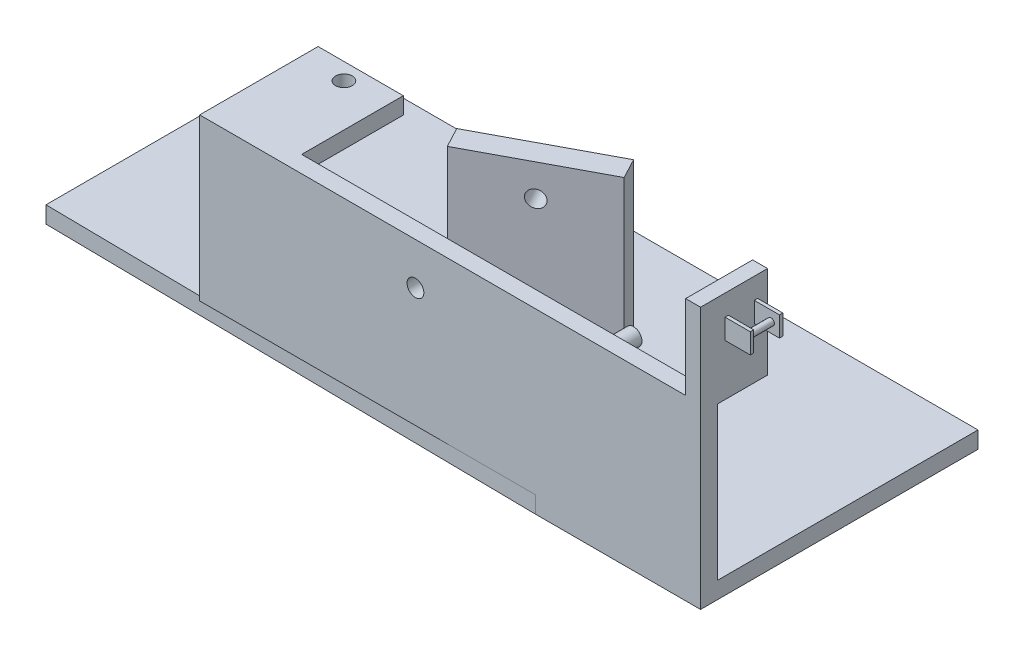
SolidWorks part; units mm, degrees
material "PBT general purpose"
ref_plane "Front Plane" through (0, 0, 0) normal (0, 0, 1) x (1, 0, 0)
ref_plane "Top Plane" through (0, 0, 0) normal (0, 1, 0) x (1, 0, 0)
ref_plane "Right Plane" through (0, 0, 0) normal (1, 0, 0) x (0, 0, -1)
sketch "Sketch1" plane through (0, 0, 0) normal (0, 1, 0) x (1, 0, 0)
  line L0 (-110.4399, 19.8241) -> (89.5601, 19.8241)
  line L1 (-120.4399, -55.1759) -> (99.5601, -55.1759)
  line L2 (-120.4399, -55.1759) -> (-120.4399, 29.8241)
  line L3 (-120.4399, 29.8241) -> (99.5601, 29.8241)
  line L4 (99.5601, -55.1759) -> (99.5601, 29.8241)
  line L5 (89.5601, -45.1759) -> (89.5601, 19.8241)
  line L6 (-110.4399, -45.1759) -> (89.5601, -45.1759)
  line L7 (-110.4399, -45.1759) -> (-110.4399, 19.8241)
  dimension "D2" = 65
  dimension "D3" = 200
  dimension "D1" = 10
extrude "Boss-Extrude1" add sketch "Sketch1" along normal blind 50
sketch "Sketch2" plane through (0, 0, 55.1759) normal (0, 0, 1) x (1, 0, 0)
  line L0 (-120.4399, 50) -> (-120.4399, 0) construction
  circle A0 centre (-70.4399, 25) radius 5
  point P2 (-120.4399, 25)
  dimension "D1" = 10
  dimension "D2" = 50
extrude "Cut-Extrude1" cut sketch "Sketch2" against normal up to surface (85 mm away) up to face at (-10.4399, 25, -29.8241)
sketch "Sketch3" plane through (0, 0, 55.1759) normal (0, 0, 1) x (1, 0, 0)
  circle A0 centre (-16.4399, 25) radius 5
  circle A1 centre (-70.4399, 25) radius 5 construction
  dimension "D1" = 10
  dimension "D2" = 54
extrude "Boss-Extrude2" add sketch "Sketch3" against normal up to surface (75 mm away) up to face at (-65.4399, 25, -19.8241)
sketch "Sketch4" plane through (0, 0, 55.1759) normal (0, 0, 1) x (1, 0, 0)
  line L0 (-120.4399, 50) -> (-120.4399, 87.8143)
  line L1 (-120.4399, 87.8143) -> (-48.8108, 87.8143)
  line L2 (-48.8108, 87.8143) -> (-48.8108, 77.8143)
  line L3 (-48.8108, 77.8143) -> (-110.4399, 77.8143)
  line L4 (-110.4399, 77.8143) -> (-110.4399, 50)
  line L5 (-120.4399, 50) -> (99.5601, 50) construction
  line L6 (-110.4399, 50) -> (-120.4399, 50)
  dimension "D1" = 10
  dimension "D2" = 10
extrude "Boss-Extrude3" add sketch "Sketch4" against normal up to surface (85 mm away) up to face at (-65.4399, 25, -29.8241)
sketch "Sketch7" plane through (0, 0, 55.1759) normal (0, 0, 1) x (1, 0, 0)
  line L0 (-120.4399, 0) -> (99.5601, 0) construction
  line L1 (-110.4399, 0) -> (99.5601, 0)
  line L2 (-110.4399, 0) -> (-110.4399, 50)
  line L3 (-110.4399, 50) -> (99.5601, 50)
  line L4 (99.5601, 0) -> (99.5601, 50)
extrude "Cut-Extrude3" cut sketch "Sketch7" against normal blind 35
sketch "Sketch8" plane through (89.5601, 0, 0) normal (-1, 0, 0) x (0, 0, 1)
  line L0 (20.1759, 50) -> (-19.8241, 50) construction
  line L1 (20.1759, 0) -> (10.1759, 0)
  line L2 (20.1759, 0) -> (20.1759, 50)
  line L3 (20.1759, 50) -> (10.1759, 50)
  line L4 (10.1759, 0) -> (10.1759, 50)
  dimension "D1" = 10
extrude "Boss-Extrude4" add sketch "Sketch8" along normal up to surface (200 mm away) up to face at (-110.4399, 42.6048, 1.0092)
sketch "Sketch9" plane through (0, 0, 0) normal (0, -1, 0) x (1, 0, 0)
  line L0 (-110.4399, 20.1759) -> (99.5601, 20.1759) construction
  line L1 (99.5601, -29.8241) -> (24.7244, -29.8241)
  line L2 (99.5601, -29.8241) -> (99.5601, 20.1759)
  line L3 (99.5601, 20.1759) -> (24.7244, 20.1759)
  line L4 (24.7244, -29.8241) -> (24.7244, 20.1759)
extrude "Boss-Extrude5" add sketch "Sketch9" against normal blind 5
sketch "Sketch10" plane through (0, 50, 0) normal (0, 1, 0) x (1, 0, 0)
  line L0 (99.5601, 29.8241) -> (-110.4399, 29.8241) construction
  line L1 (99.5601, -20.1759) -> (46.5233, -20.1759)
  line L2 (99.5601, -20.1759) -> (99.5601, 29.8241)
  line L3 (99.5601, 29.8241) -> (46.5233, 29.8241)
  line L4 (46.5233, -20.1759) -> (46.5233, -2.1759)
  line L5 (46.5233, -2.1759) -> (54.5601, -2.1759)
  line L6 (54.5601, -2.1759) -> (54.5601, 9.8241)
  line L7 (54.5601, 9.8241) -> (46.5233, 9.8241)
  line L8 (46.5233, 9.8241) -> (46.5233, 29.8241)
  dimension "D1" = 18
  dimension "D2" = 12
  dimension "D3" = 45
extrude "Boss-Extrude6" add sketch "Sketch10" against normal blind 5
sketch "Sketch11" plane through (0, 50, 0) normal (0, 1, 0) x (1, 0, 0)
  line L0 (99.5601, 29.8241) -> (-110.4399, 29.8241) construction
  line L1 (99.5601, -20.1759) -> (63.4572, -20.1759)
  line L2 (99.5601, -20.1759) -> (99.5601, 29.8241)
  line L3 (99.5601, 29.8241) -> (63.4572, 29.8241)
  line L4 (63.4572, -20.1759) -> (63.4572, 29.8241)
extrude "Cut-Extrude4" cut sketch "Sketch11" against normal through all
sketch "Sketch12" plane through (0, 50, 0) normal (0, 1, 0) x (1, 0, 0)
  line L0 (63.4572, 29.8241) -> (63.4572, -20.1759) construction
  line L1 (46.5233, -10.1759) -> (63.4572, -10.1759)
  line L2 (46.5233, -10.1759) -> (46.5233, -2.1759)
  line L3 (46.5233, 19.755) -> (63.4572, 19.755)
  line L4 (63.4572, -10.1759) -> (63.4572, 19.755)
  line L5 (46.5233, 9.8241) -> (46.5233, 19.755)
  line L6 (54.5601, -2.1759) -> (46.5233, -2.1759)
  line L7 (54.5601, -2.1759) -> (54.5601, 9.8241)
  line L8 (54.5601, 9.8241) -> (46.5233, 9.8241)
extrude "Boss-Extrude7" add sketch "Sketch12" along normal blind 50
sketch "Sketch13" plane through (0, 0, 0) normal (0, -1, 0) x (1, 0, 0)
  line L0 (-120.4399, 55.1759) -> (-120.4399, 105.1759)
  line L2 (-110.4399, 108.1048) -> (-62.671, 155.8738)
  line L3 (-62.671, 155.8738) -> (-66.2065, 159.4093)
  line L4 (-110.4399, 108.1048) -> (-110.4399, 55.1759)
  line L5 (-48.8108, 55.1759) -> (-120.4399, 55.1759) construction
  line L6 (-110.4399, 55.1759) -> (-120.4399, 55.1759)
  line L7 (-66.2065, 159.4093) -> (-120.4399, 105.1759)
  dimension "D1" = 5
  dimension "D2" = 10
  dimension "D3" = 135
extrude "Boss-Extrude8" add sketch "Sketch13" against normal blind 50 separate body
sketch "Sketch14" plane through (0, 0, 10.1759) normal (0, 0, -1) x (-1, 0, 0)
  circle A0 centre (70.4399, 25) radius 4.9995
extrude "Cut-Extrude5" cut sketch "Sketch14" against normal blind 50
sketch "Sketch17" plane through (0, 0, 0) normal (0, -1, 0) x (1, 0, 0)
  line L0 (24.7244, -19.8241) -> (-110.4399, -19.8241) construction
  line L1 (63.4572, -29.8241) -> (-110.4399, -29.8241)
  line L2 (63.4572, -29.8241) -> (63.4572, -19.8241)
  line L3 (63.4572, -19.8241) -> (-110.4399, -19.8241)
  line L4 (-110.4399, -29.8241) -> (-110.4399, -19.8241)
extrude "Cut-Extrude7" cut sketch "Sketch17" against normal up to next (50 mm away)
sketch "Sketch18" plane through (-109.2724, 0, 109.2724) normal (0.7071, 0, -0.7071) x (-0.7071, 0, -0.7071)
  line L0 (1.6512, 0) -> (-65.9043, 0) construction
  circle A0 centre (-32.1266, 25) radius 5
  dimension "D1" = 10
  dimension "D2" = 25
extrude "Cut-Extrude8" cut sketch "Sketch18" against normal blind 10
sketch "Sketch20" plane through (0, 87.8143, 0) normal (0, 1, 0) x (1, 0, 0)
  circle A0 centre (-70.1737, -35.2467) radius 5
extrude "Cut-Extrude9" cut sketch "Sketch20" against normal blind 15
sketch "Sketch23" plane through (0, 0, 0) normal (0, -1, 0) x (1, 0, 0)
  line L1 (24.7244, 10.1759) -> (63.4572, 10.1759)
  line L2 (24.7244, 10.1759) -> (24.7244, -19.8241)
  line L3 (24.7244, -19.8241) -> (63.4572, -19.8241)
  line L4 (63.4572, 10.1759) -> (63.4572, -19.8241)
extrude "Cut-Extrude12" cut sketch "Sketch23" against normal blind 15
sketch "Sketch24" plane through (-110.4399, 0, 0) normal (1, 0, 0) x (0, 0, -1)
  line L1 (-178.5753, 76.7479) -> (-55.1759, 76.7479)
  line L2 (-178.5753, 76.7479) -> (-178.5753, 0)
  line L3 (-178.5753, 0) -> (-55.1759, 0)
  line L4 (-55.1759, 76.7479) -> (-55.1759, 0)
extrude "Cut-Extrude14" cut sketch "Sketch24" against normal mid plane 100
sketch "Sketch26" plane through (0, 0, 0) normal (0, -1, 0) x (1, 0, 0)
  line L0 (-120.4399, -29.8241) -> (-120.4399, -82.8241)
  line L1 (-110.4399, -29.8241) -> (-110.4399, -82.8241)
  line L2 (-110.4399, -82.8241) -> (-60.5112, -132.7528)
  line L3 (-120.4399, -82.8241) -> (-64.6115, -138.6525)
  line L4 (-64.6115, -138.6525) -> (-60.5112, -132.7528)
  line L5 (-120.4399, -29.8241) -> (-110.4399, -29.8241)
extrude "Boss-Extrude9" add sketch "Sketch26" against normal blind 60
sketch "Sketch27" plane through (-96.632, 0, -96.632) normal (0.7071, 0, 0.7071) x (0.7071, 0, -0.7071)
  circle A0 centre (14.4727, 25) radius 5
extrude "Cut-Extrude15" cut sketch "Sketch27" against normal blind 60
sketch "Sketch28" plane through (63.4572, 0, 0) normal (1, 0, 0) x (0, 0, -1)
  line L4 (-3.5599, 87.5411) -> (-5.5599, 87.5411)
  line L5 (-5.5599, 87.5411) -> (-5.5599, 75.5411)
  line L6 (-3.5599, 87.5411) -> (-3.5599, 75.5411)
  line L7 (-3.5599, 75.5411) -> (-5.5599, 75.5411)
  line L8 (11.8241, 87.5411) -> (13.8241, 87.5411)
  line L9 (13.8241, 87.5411) -> (13.8241, 75.5411)
  line L10 (13.8241, 75.5411) -> (11.8241, 75.5411)
  line L11 (11.8241, 75.5411) -> (11.8241, 87.5411)
extrude "Boss-Extrude10" add sketch "Sketch28" along normal blind 15
sketch "Sketch29" plane through (0, 0, 5.5599) normal (0, 0, 1) x (1, 0, 0)
  circle A0 centre (73.4572, 81.5411) radius 2
extrude "Boss-Extrude11" add sketch "Sketch29" against normal blind 18
sketch "Sketch30" plane through (-48.8108, 0, 0) normal (1, 0, 0) x (0, 0, -1)
  line L0 (10.1347, 87.8143) -> (18.6732, 87.8143)
  line L1 (29.8241, 87.8143) -> (-55.1759, 87.8143) construction
  line L2 (18.6732, 87.8143) -> (14.404, 97.0575)
  line L3 (14.404, 97.0575) -> (10.1347, 87.8143)
sketch "Sketch31" plane through (0, 87.8143, 0) normal (0, 1, 0) x (1, 0, 0)
  line L0 (-48.8108, 10.1347) -> (-48.8108, 18.6732) construction
  line L1 (-120.4399, 29.8241) -> (-120.4399, -55.1759) construction
  spline S0 degree 3 poles (-48.8108, 14.404) (-68.2087, 19.7403) (-84.0911, -3.4277) (-107.8721, -25.1931) (-120.4399, -12.6759) knots 0 0 0 0 0.557371 1 1 1 1
sweep "Sweep1" add profiles "Sketch30" path "Sketch31"
sketch "Sketch32" plane through (-110.4399, 0, 0) normal (1, 0, 0) x (0, 0, -1)
  line L1 (29.8241, 60) -> (152.1894, 60)
  line L2 (29.8241, 60) -> (29.8241, -15.4022)
  line L3 (29.8241, -15.4022) -> (152.1894, -15.4022)
  line L4 (152.1894, 60) -> (152.1894, -15.4022)
extrude "Cut-Extrude16" cut sketch "Sketch32" against normal mid plane 100
sketch "Sketch33" plane through (0, 0, -9.8241) normal (0, 0, 1) x (1, 0, 0)
  line L1 (54.5601, 100) -> (46.5233, 100)
  line L2 (54.5601, 100) -> (54.5601, 45)
  line L3 (54.5601, 45) -> (46.5233, 45)
  line L4 (46.5233, 100) -> (46.5233, 45)
extrude "Cut-Extrude17" cut sketch "Sketch33" against normal mid plane 40
sketch "Sketch34" plane through (0, 0, 10.1759) normal (0, 0, 1) x (1, 0, 0)
  line L1 (54.5601, 100) -> (63.4572, 100)
  line L2 (54.5601, 100) -> (54.5601, 50)
  line L3 (54.5601, 50) -> (63.4572, 50)
  line L4 (63.4572, 100) -> (63.4572, 50)
extrude "Boss-Extrude12" add sketch "Sketch34" along normal blind 10
sketch "Sketch35" plane through (0, 0, -19.8241) normal (0, 0, -1) x (-1, 0, 0)
  line L0 (16.4399, 25) -> (16.4399, -46)
ref_plane "Plane1" through (0, -46, 0) normal (0, 1, 0) x (1, 0, 0)
sketch "Sketch36" plane through (0, -46, 0) normal (0, 1, 0) x (1, 0, 0)
  line L0 (-110.4399, -20.1759) -> (63.4572, -20.1759) construction
  line L1 (-35.0234, -20.1759) -> (63.4572, -20.1759)
  line L2 (-35.0234, -20.1759) -> (-35.0234, 30.7287)
  line L3 (-35.0234, 30.7287) -> (63.4572, 30.7287)
  line L4 (63.4572, -20.1759) -> (63.4572, 30.7287)
extrude "Boss-Extrude13" add sketch "Sketch36" against normal blind 10 separate body
sketch "Sketch37" plane through (0, -46, 0) normal (0, 1, 0) x (1, 0, 0)
  line L0 (63.4572, -20.1759) -> (63.4572, 30.7287) construction
  line L1 (-35.0234, -20.1759) -> (63.4572, -20.1759)
  line L2 (-35.0234, -20.1759) -> (-35.0234, -10.1759)
  line L3 (-35.0234, -10.1759) -> (63.4572, -10.1759)
  line L4 (63.4572, -20.1759) -> (63.4572, -10.1759)
  line L5 (-110.4399, -10.1759) -> (63.4572, -10.1759) construction
extrude "Boss-Extrude14" add sketch "Sketch37" along normal blind 46
ref_plane "Plane2" through (-35.0234, 0, 0) normal (1, 0, 0) x (0, 0, -1)
sketch "Sketch39" plane through (-35.0234, 0, 0) normal (1, 0, 0) x (0, 0, -1)
  line L1 (35.5386, 90.5816) -> (-64.8845, 90.5816)
  line L2 (35.5386, 90.5816) -> (35.5386, -58.8284)
  line L3 (35.5386, -58.8284) -> (-64.8845, -58.8284)
  line L4 (-64.8845, 90.5816) -> (-64.8845, -58.8284)
extrude "Cut-Extrude21" cut sketch "Sketch39" against normal blind 100
sketch "Sketch40" plane through (-35.0234, 0, 0) normal (1, 0, 0) x (0, 0, -1)
  line L1 (-73.704, 85.0863) -> (47.7926, 85.0863)
  line L2 (-73.704, 85.0863) -> (-73.704, 128.8491)
  line L3 (-73.704, 128.8491) -> (47.7926, 128.8491)
  line L4 (47.7926, 85.0863) -> (47.7926, 128.8491)
extrude "Cut-Extrude22" cut sketch "Sketch40" against normal blind 100
ref_plane "Plane3" through (0, -56, 0) normal (0, 1, 0) x (1, 0, 0)
sketch "Sketch41" plane through (0, -56, 0) normal (0, 1, 0) x (1, 0, 0)
  line L0 (-35.0234, -20.1759) -> (-556.5938, -13.4122)
  line L1 (-556.5938, -13.4122) -> (-556.5938, 189.172)
  line L2 (-556.5938, 189.172) -> (63.4572, 189.172)
  line L3 (63.4572, 189.172) -> (63.4572, 30.7287)
  line L4 (63.4572, 30.7287) -> (-34.3633, 30.7287)
  line L5 (-34.3633, 30.7287) -> (-35.0234, -20.1759)
extrude "Boss-Extrude15" add sketch "Sketch41" along normal blind 10
sketch "Sketch42" plane through (-35.0234, 0, 0) normal (-1, 0, 0) x (0, 0, 1)
  line L1 (10.1759, 50) -> (20.1759, 50)
  line L2 (10.1759, 50) -> (10.1759, -46)
  line L3 (10.1759, -46) -> (20.1759, -46)
  line L4 (20.1759, 50) -> (20.1759, -46)
extrude "Boss-Extrude17" add sketch "Sketch42" along normal blind 200
sketch "Sketch44" plane through (0, 0, 10.1759) normal (0, 0, -1) x (-1, 0, 0)
  circle A0 centre (106.4399, 25) radius 5
extrude "Cut-Extrude24" cut sketch "Sketch44" against normal blind 200
sketch "Sketch47" plane through (0, 50, 0) normal (0, 1, 0) x (1, 0, 0)
  line L1 (-235.0234, -10.1759) -> (-184.2514, -10.1759)
  line L2 (-235.0234, -10.1759) -> (-235.0234, 50.3973)
  line L3 (-235.0234, 50.3973) -> (-184.2514, 50.3973)
  line L4 (-184.2514, -10.1759) -> (-184.2514, 50.3973)
extrude "Boss-Extrude19" add sketch "Sketch47" against normal blind 10
sketch "Sketch48" plane through (0, 50, 0) normal (0, 1, 0) x (1, 0, 0)
  circle A0 centre (-209.6374, 40.3973) radius 5
extrude "Cut-Extrude26" cut sketch "Sketch48" against normal blind 10
sketch "Sketch49" plane through (0, -46, 0) normal (0, 1, 0) x (1, 0, 0)
  line L0 (-157.3869, 55.3837) -> (-151.0035, 43.3906)
  line L1 (-151.0035, 43.3906) -> (-94.2648, 73.59)
  line L2 (-88.6197, 91.9854) -> (-82.2362, 79.9923)
  line L3 (-100.6482, 85.5832) -> (-157.3869, 55.3837)
  line L4 (-100.6482, 85.5832) -> (-88.6197, 91.9854)
  line L5 (-82.2362, 79.9923) -> (-94.2648, 73.59)
sketch "Sketch51" plane through (0, -46, 0) normal (0, 1, 0) x (1, 0, 0)
  line L0 (-556.5938, -13.4122) -> (-235.0234, -17.5823) construction
  line L1 (-556.5938, 189.172) -> (-330.4253, 189.172)
  line L2 (-556.5938, 189.172) -> (-556.5938, -16.3452)
  line L3 (-556.5938, -16.3452) -> (-330.4253, -16.3452)
  line L4 (-330.4253, 189.172) -> (-330.4253, -16.3452)
extrude "Cut-Extrude28" cut sketch "Sketch51" against normal blind 30
extrude "Boss-Extrude22" add sketch "Sketch49" along normal blind 90
sketch "Sketch52" plane through (-57.7148, 0, -108.4346) normal (-0.4698, 0, -0.8827) x (-0.8827, 0, 0.4698)
  circle A0 centre (73.9604, 25) radius 5
extrude "Cut-Extrude29" cut sketch "Sketch52" against normal blind 30
sketch "Sketch53" plane through (0, -46, 0) normal (0, 1, 0) x (1, 0, 0)
  line L0 (63.4572, -10.1759) -> (63.4572, 189.172) construction
  line L1 (-330.4253, 189.172) -> (63.4572, 189.172)
  line L2 (-330.4253, 189.172) -> (-330.4253, 145.1542)
  line L3 (-330.4253, 145.1542) -> (63.4572, 145.1542)
  line L4 (63.4572, 189.172) -> (63.4572, 145.1542)
extrude "Cut-Extrude30" cut sketch "Sketch53" against normal blind 30
